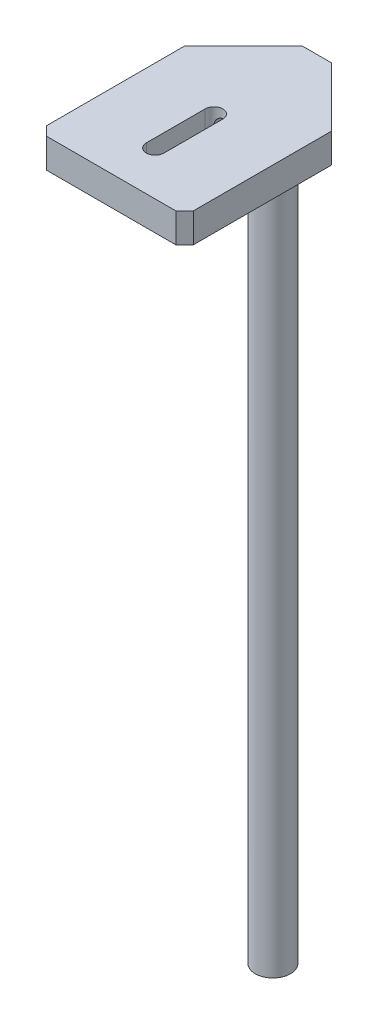
SolidWorks part; units mm, degrees
ref_plane "Front Plane" through (0, 0, 0) normal (0, 0, 1) x (1, 0, 0)
ref_plane "Top Plane" through (0, 0, 0) normal (0, 1, 0) x (1, 0, 0)
ref_plane "Right Plane" through (0, 0, 0) normal (1, 0, 0) x (0, 0, -1)
sketch "Sketch1" plane through (0, 0, 0) normal (0, 1, 0) x (1, 0, 0)
  line L0 (-25, 25) -> (-5, 45)
  line L1 (-25, -25) -> (25, -25)
  line L2 (-25, -25) -> (-25, 25)
  line L4 (25, -25) -> (25, 25)
  line L5 (-25, -25) -> (25, 25) construction
  line L6 (-25, 25) -> (25, -25) construction
  line L7 (-5, 45) -> (5, 45)
  line L8 (5, 45) -> (25, 25)
  point P0 (0, 0)
  dimension "D1" = 50
  dimension "D2" = 50
  dimension "D3" = 70
  dimension "D4" = 10
extrude "Boss-Extrude1" add sketch "Sketch1" along normal blind 10
sketch "Sketch2" plane through (0, 10, 0) normal (0, -1, 0) x (1, 0, 0)
  line L0 (5, -45) -> (-5, -45) construction
  line L1 (0, -45) -> (0, -30) construction
  circle A0 centre (0, -30) radius 6
  dimension "D1" = 12
  dimension "D2" = 15
extrude "Boss-Extrude2" add sketch "Sketch2" along normal blind 260
sketch "Sketch3" plane through (0, 0, 0) normal (0, -1, 0) x (1, 0, 0)
  line L0 (0, -10) -> (0, 10) construction
  line L1 (-3, -10) -> (-3, 10)
  line L2 (3, -10) -> (3, 10)
  arc A0 (-3, -10) -> (3, -10) centre (0, -10) ccw
  arc A1 (3, 10) -> (-3, 10) centre (0, 10) ccw
  point P3 (0, 0)
  dimension "D1" = 6
  dimension "D2" = 20
extrude "Cut-Extrude1" cut sketch "Sketch3" against normal through all
sketch "Sketch4" plane through (0, 10, 0) normal (0, 1, 0) x (1, 0, 0)
  circle A0 centre (0, 30) radius 6
  dimension "D1" = 12
extrude "Cut-Extrude2" [suppressed] cut sketch "Sketch4" against normal blind 10
hole_wizard "M5 Tapped Hole1" positions "Sketch5" profile "Sketch6" tap size "M5" standard "GB"
sketch "Sketch5" plane through (0, 0, -45) normal (0, 0, -1) x (-1, 0, 0)
  line L0 (5, 10) -> (5, 0) construction
  line L1 (-5, 10) -> (5, 10) construction
  point P0 (0, 5)
  dimension "D1" = 5
  dimension "D2" = 5
cosmetic thread "Hole thread line1" parameters "D1"=32.9, "D2"=5
sketch "Sketch6" plane through (0, 5, -45) normal (1, 0, 0) x (0, 1, 0)
  line L0 (0, 0) -> (0, 38.1618)
  line L1 (0, 38.1618) -> (2.1, 36.9)
  line L2 (2.1, 36.9) -> (2.1, 0)
  line L5 (2.1, 0) -> (0, 0)
  line L10 (0, 38.1618) -> (-2.1, 36.9) construction
  line L11 (0, -6.35) -> (0, 107.95) construction
  dimension "螺纹孔钻头直径" = 4.2
  dimension "螺纹孔钻头深度" = 36.9
  dimension "导头角度" = 118
chamfer "Chamfer1" distance 3 angle 45 2 edges at (-25, 5, 25) (25, 5, 25)
equation "\"1\"= \"代号代号\""
equation "\"2\"= \"名称代号\""
